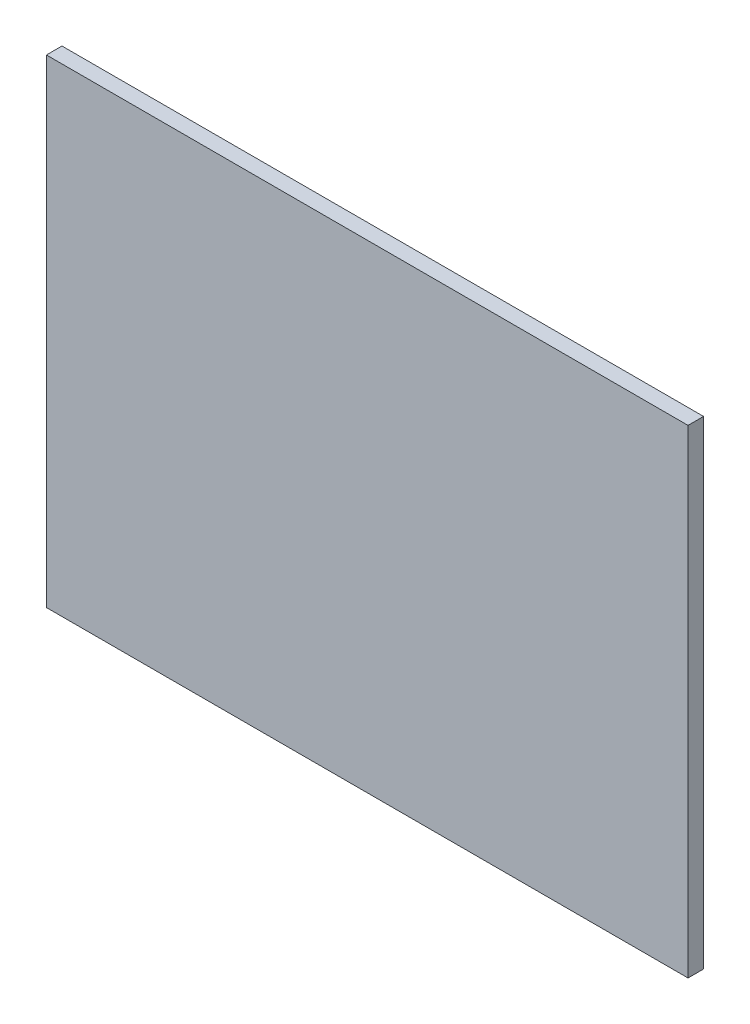
from build123d import *

# Parameters (mm, degrees)
SKETCH_1_W      = 248
SKETCH_1_H      = 185
EXTRUDE_1_DEPTH = 6


with BuildPart() as part:
    # 草图1 → 凸台-拉伸1 (new body)
    with BuildSketch(Plane.XY):
        Rectangle(SKETCH_1_W, SKETCH_1_H)
    extrude(amount=EXTRUDE_1_DEPTH)


solid = part.part
